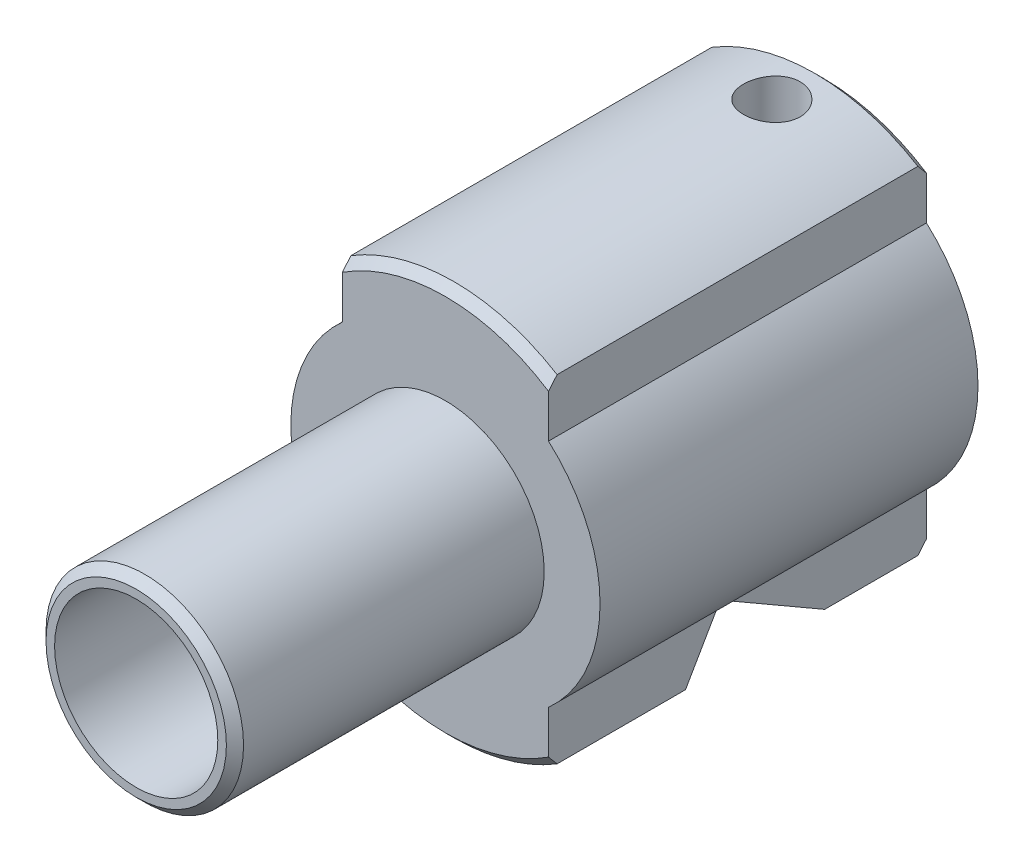
SolidWorks part; units mm, degrees
ref_plane "Front Plane" through (0, 0, 0) normal (0, 0, 1) x (1, 0, 0)
ref_plane "Top Plane" through (0, 0, 0) normal (0, 1, 0) x (1, 0, 0)
ref_plane "Right Plane" through (0, 0, 0) normal (1, 0, 0) x (0, 0, -1)
sketch "Sketch1" plane through (0, 0, 0) normal (0, 0, 1) x (1, 0, 0)
  circle A0 centre (0, 0) radius 4.75
  circle A1 centre (0, 0) radius 11.5
  dimension "D1" = 9.5
  dimension "D2" = 23
extrude "Boss-Extrude1" add sketch "Sketch1" along normal blind 22
sketch "Sketch2" plane through (0, 0, 22) normal (0, 0, 1) x (1, 0, 0)
  circle A0 centre (0, 0) radius 4.75 construction
  circle A1 centre (0, 0) radius 4.75
  circle A2 centre (0, 0) radius 5.75
  dimension "D1" = 11.5
extrude "Boss-Extrude2" add sketch "Sketch2" along normal blind 18
sketch "Sketch3" plane through (0, 0, 0) normal (0, 0, -1) x (-1, 0, 0)
  circle A0 centre (0, 0) radius 6.5
  dimension "D1" = 13
extrude "Cut-Extrude1" cut sketch "Sketch3" against normal blind 8
chamfer "Chamfer1" distance 0.5 angle 45 2 edges at (11.5, 0, 22) (11.5, 0, 0)
hole_wizard "M4 Tapped Hole3" positions "Sketch13" profile "Sketch12" tap size "M4" standard "Gb"
sketch "Sketch13" plane through (0, 0, 0) normal (0, 1, 0) x (1, 0, 0)
  line L0 (6.5, 0) -> (-6.5, 0) construction
  point P0 (0, -3)
  dimension "D1" = 3
sketch "Sketch12" plane through (0, 0, 3) normal (1, 0, 0) x (0, 0, -1)
  line L0 (0, 0) -> (0, 11.5)
  line L1 (0, 11.5) -> (1.65, 11.5)
  line L2 (1.65, 11.5) -> (1.65, 0)
  line L5 (1.65, 0) -> (0, 0)
  line L11 (0, -6.35) -> (0, 107.95) construction
  dimension "通孔螺纹孔钻头直径" = 3.3
  dimension "通孔螺纹孔钻头深度" = 11.5
cosmetic thread "Hole Thread4" parameters "D2"=4
sketch "Sketch14" plane through (0, 0, 0) normal (1, 0, 0) x (0, 0, -1)
  line L0 (-15, -11.5) -> (-12, -6.3038)
  line L1 (-12, -6.3038) -> (-3, -11.5)
  line L2 (-21.5, -11.5) -> (-0.5, -11.5) construction
  line L3 (-15, -11.5) -> (-3, -11.5)
  line L4 (-22, 11) -> (-22, -11) construction
  dimension "D1" = 30
  dimension "D2" = 7
  dimension "D3" = 12
extrude "Cut-Extrude4" cut sketch "Sketch14" against normal through all and the other way through all
hole_wizard "Ø1.2 (1.2) Diameter Hole1" positions "Sketch16" profile "Sketch15" hole size "Ø1.2" standard "Gb"
sketch "Sketch16" plane through (0, 3.6202, 6.2704) normal (0, -0.5, -0.866) x (-1, 0, 0)
  line L0 (9.6183, -11.4593) -> (-9.6183, -11.4593) construction
  point P0 (0, -14.4593)
  dimension "D1" = 3
sketch "Sketch15" plane through (0, -8.9019, 13.5) normal (1, 0, 0) x (0, 0.866, -0.5)
  line L0 (0, 0) -> (0, 8.3038)
  line L1 (0, 8.3038) -> (0.6, 8.3038)
  line L2 (0.6, 8.3038) -> (0.6, 0)
  line L5 (0.6, 0) -> (0, 0)
  line L11 (0, -6.35) -> (0, 107.95) construction
  dimension "通孔孔直径" = 1.2
  dimension "通孔孔深度" = 8.3038
hole_wizard "M3 Tapped Hole2" positions "Sketch18" profile "Sketch17" tap size "M3" standard "Gb"
sketch "Sketch18" plane through (0, 3.6202, 6.2704) normal (0, -0.5, -0.866) x (-1, 0, 0)
  point P0 (0, -14.4593)
sketch "Sketch17" plane through (0, -8.9019, 13.5) normal (1, 0, 0) x (0, 0.866, -0.5)
  line L0 (0, 0) -> (0, 5.2511)
  line L1 (0, 5.2511) -> (1.25, 4.5)
  line L2 (1.25, 4.5) -> (1.25, 0)
  line L5 (1.25, 0) -> (0, 0)
  line L10 (0, 5.2511) -> (-1.25, 4.5) construction
  line L11 (0, -6.35) -> (0, 107.95) construction
  dimension "螺纹孔钻头直径" = 2.5
  dimension "螺纹孔钻头深度" = 4.5
  dimension "导头角度" = 118
cosmetic thread "Hole Thread5" parameters "D1"=3, "D2"=3
chamfer "Chamfer2" distance 0.3 distance2 8 1 edges at (-4.75, 0, 8)
sketch "Sketch19" plane through (0, 0, 0) normal (0, 0, -1) x (-1, 0, 0)
  line L0 (0, 0) -> (0, 12.56) construction
  line L1 (-6, 9.8107) -> (-6, 6.7082)
  line L2 (6, 9.8107) -> (6, 6.7082)
  line L3 (-6, -6.7082) -> (-6, -9.8107)
  line L4 (6, -6.7082) -> (6, -9.8107)
  circle A1 centre (0, 0) radius 11.5 construction
  arc A2 (6, -9.8107) -> (6, 9.8107) centre (0, 0) ccw
  arc A3 (6, -6.7082) -> (6, 6.7082) centre (0, 0) ccw
  arc A4 (-6, 6.7082) -> (-6, -6.7082) centre (0, 0) ccw
  arc A5 (-6, 9.8107) -> (-6, -9.8107) centre (0, 0) ccw
  dimension "D1" = 18
  dimension "D2" = 12
extrude "Cut-Extrude5" cut sketch "Sketch19" against normal through all
chamfer "Chamfer3" distance 0.5 angle 45 2 edges at (-6.5, 0, 0) (5.75, 0, 40)
